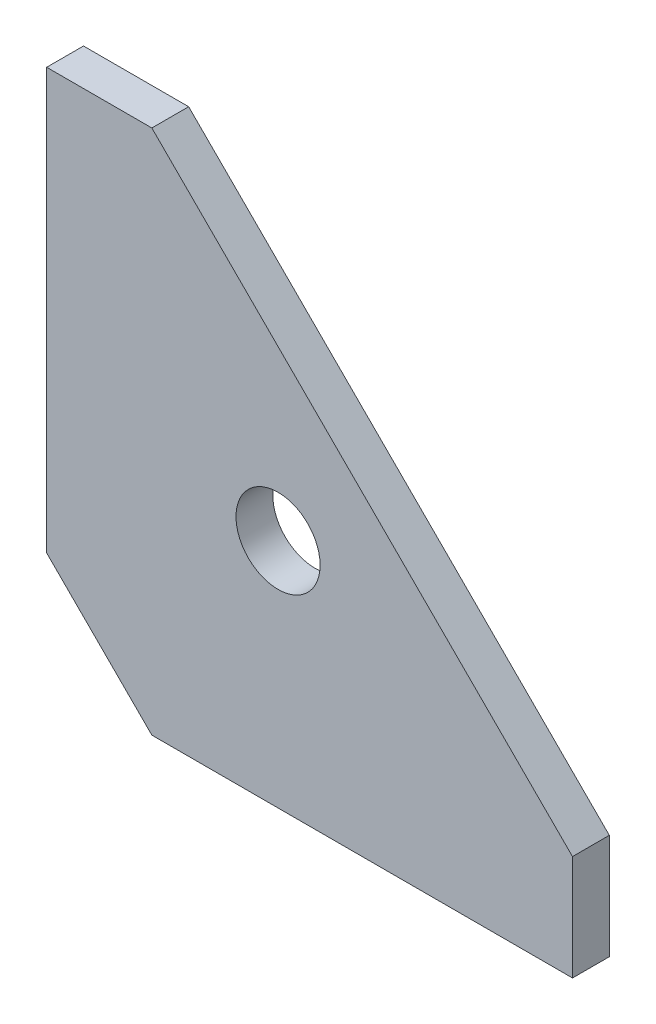
SolidWorks part; units mm, degrees
material "普通碳钢"
ref_plane "Front Plane" through (0, 0, 0) normal (0, 0, 1) x (1, 0, 0)
ref_plane "Top Plane" through (0, 0, 0) normal (0, 1, 0) x (1, 0, 0)
ref_plane "Right Plane" through (0, 0, 0) normal (1, 0, 0) x (0, 0, -1)
sketch "Sketch1" plane through (0, 0, 0) normal (0, 0, 1) x (1, 0, 0)
  line L0 (0, 0) -> (40, 0)
  line L1 (40, 0) -> (200, -160)
  line L2 (200, -160) -> (200, -200)
  line L3 (200, -200) -> (40, -200)
  line L4 (40, -200) -> (0, -160)
  line L5 (0, -160) -> (0, 0)
  circle A0 centre (88, -112) radius 16
  dimension "D9" = 32
  dimension "D1" = 200
  dimension "D2" = 40
  dimension "D3" = 40
  dimension "D4" = 160
  dimension "D5" = 40
  dimension "D6" = 40
  dimension "D7" = 88
  dimension "D8" = 88
extrude "Boss-Extrude1" add sketch "Sketch1" along normal blind 14
